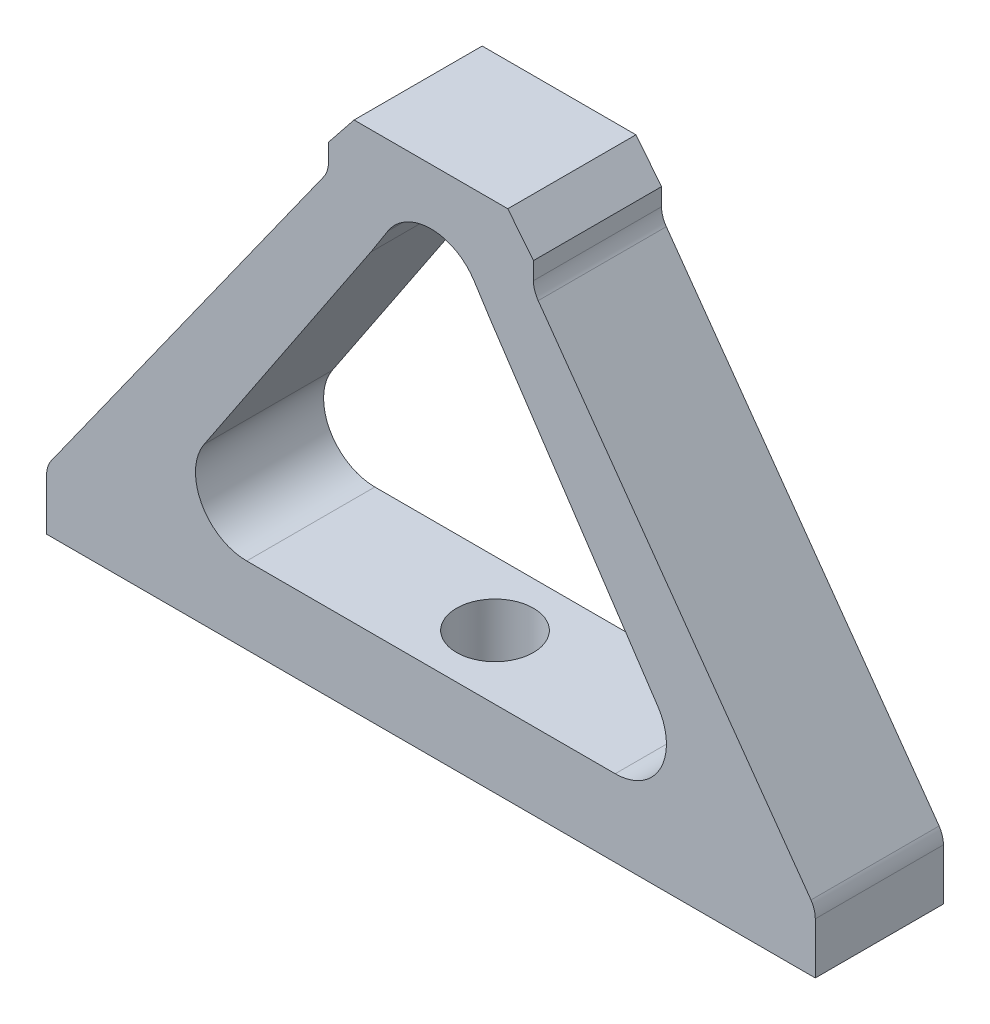
from build123d import *

# Parameters (mm, degrees)
EXTRUDE_1_DEPTH     = 10
SKETCH_3_R          = 3
CUT_EXTRUDE_1_DEPTH = 10


with BuildPart() as part:
    # 草图1 → 凸台-拉伸1 (new body)
    with BuildSketch(Plane.XY):
        with BuildLine():
            Line((-36.484728771, -19.952952756), (23.515271229, -19.952952756))
            Line((23.515271229, -19.952952756), (23.515271229, -15.952952756))
            ThreePointArc((23.515271229, -15.952952756), (23.429409838, -15.373234389), (23.179197844, -14.843291448))
            Line((23.179197844, -14.843291448), (1.886808682, 15.02014861))
            ThreePointArc((1.886808682, 15.02014861), (1.61041886, 15.571691167), (1.515271229, 16.181229888))
            Line((1.515271229, 16.181229888), (1.515271229, 17.541244626))
            Line((1.515271229, 17.541244626), (-0.484728771, 20.047047244))
            Line((-0.484728771, 20.047047244), (-12.484728771, 20.047047244))
            Line((-12.484728771, 20.047047244), (-14.484728771, 17.541244626))
            Line((-14.484728771, 17.541244626), (-14.484728771, 16.181229888))
            ThreePointArc((-14.484728771, 16.181229888), (-14.579876402, 15.571691167), (-14.856266224, 15.02014861))
            Line((-14.856266224, 15.02014861), (-36.148451723, -14.842986118))
            ThreePointArc((-36.148451723, -14.842986118), (-36.39881418, -15.373058759), (-36.484728771, -15.952952756))
            Line((-36.484728771, -15.952952756), (-36.484728771, -19.952952756))
        make_face()
        with BuildLine():
            Line((-24.192238855, -7.733019479), (-11.181735098, 11.768353778))
            Line((-11.181735098, 11.768353778), (-9.853193624, 13.848209774))
            ThreePointArc((-9.853193624, 13.848209774), (-6.483571586, 15.694946417), (-3.112703027, 13.850486044))
            Line((-3.112703027, 13.850486044), (-1.802931634, 11.803064426))
            Line((-1.802931634, 11.803064426), (11.2259567, -7.733630139))
            ThreePointArc((11.2259567, -7.733630139), (11.424949828, -11.840107961), (7.89810347, -13.952952756))
            Line((7.89810347, -13.952952756), (-20.864792951, -13.952952756))
            ThreePointArc((-20.864792951, -13.952952756), (-24.391812451, -11.839784346), (-24.192238855, -7.733019479))
        make_face(mode=Mode.SUBTRACT)
    extrude(amount=EXTRUDE_1_DEPTH)

    # 草图3 → 切除-拉伸1 (cut)
    with BuildSketch(Plane.XZ.offset(19.952952756)):
        with Locations((-6.484728771, 5)):
            Circle(SKETCH_3_R)
    extrude(amount=-CUT_EXTRUDE_1_DEPTH, mode=Mode.SUBTRACT)


solid = part.part
